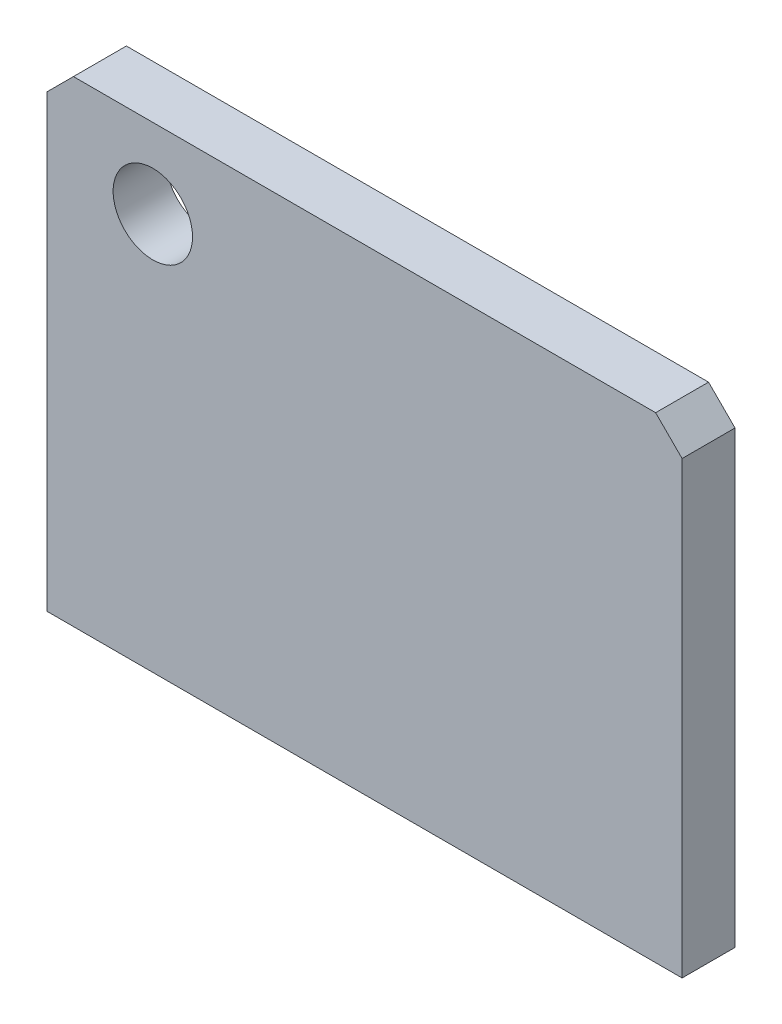
from build123d import *

# Parameters (mm, degrees)
SKETCH1_W           = 120
SKETCH1_H           = 90
BOSS_EXTRUDE1_DEPTH = 10
SKETCH2_R           = 7.5
CUT_EXTRUDE1_DEPTH  = 10
CHAMFER1_SIZE       = 5


with BuildPart() as part:
    # Sketch1 → Boss-Extrude1 (new body)
    with BuildSketch(Plane.XY):
        Rectangle(SKETCH1_W, SKETCH1_H)
    extrude(amount=BOSS_EXTRUDE1_DEPTH)

    # Sketch2 → Cut-Extrude1 (cut)
    with BuildSketch(Plane.XY.offset(10)):
        with Locations((-40, 30)):
            Circle(SKETCH2_R)
    extrude(amount=-CUT_EXTRUDE1_DEPTH, mode=Mode.SUBTRACT)

    # Chamfer1
    chamfer1_edges = [part.edges().sort_by_distance(p)[0] for p in [
        (-60, 45, 5),
        (60, 45, 5),
    ]]
    chamfer(chamfer1_edges, length=CHAMFER1_SIZE)


solid = part.part
